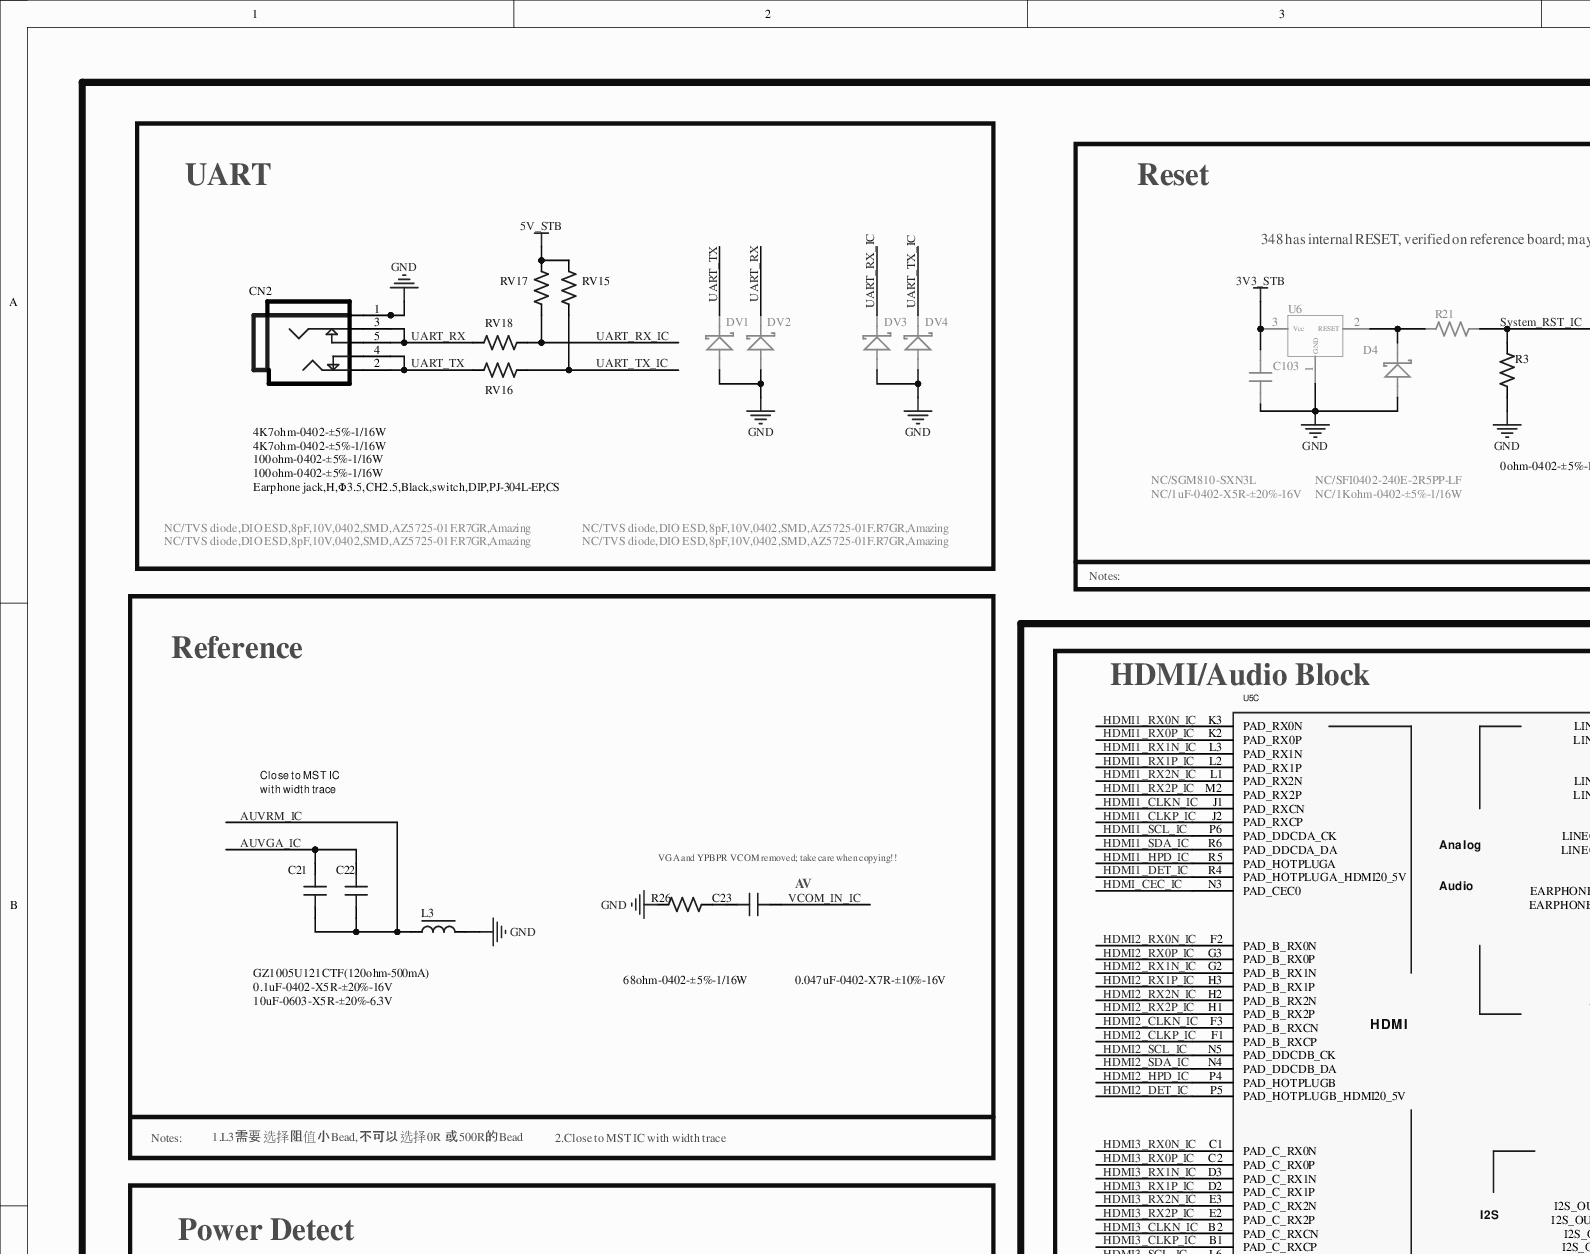
[diagram p0: MISC84395-8.SchDoc, top left]
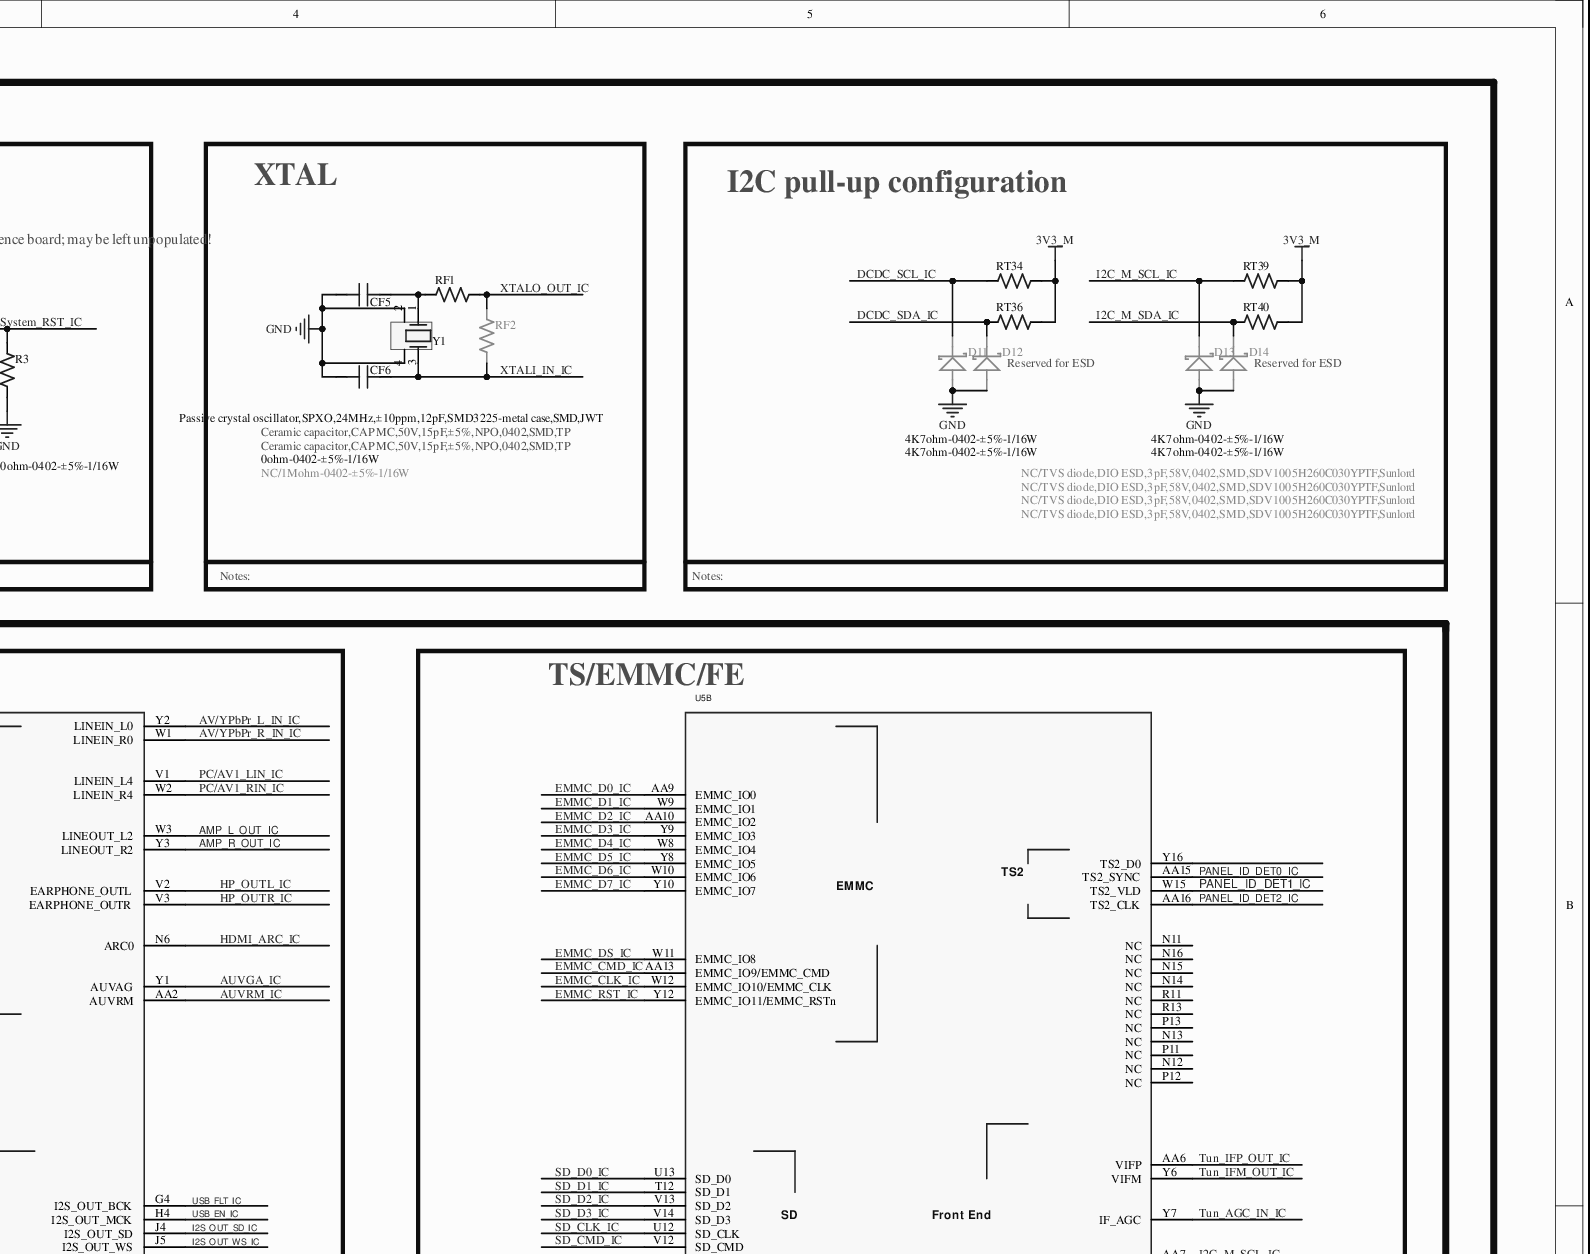
[diagram p1: MISC84395-8.SchDoc, top right]
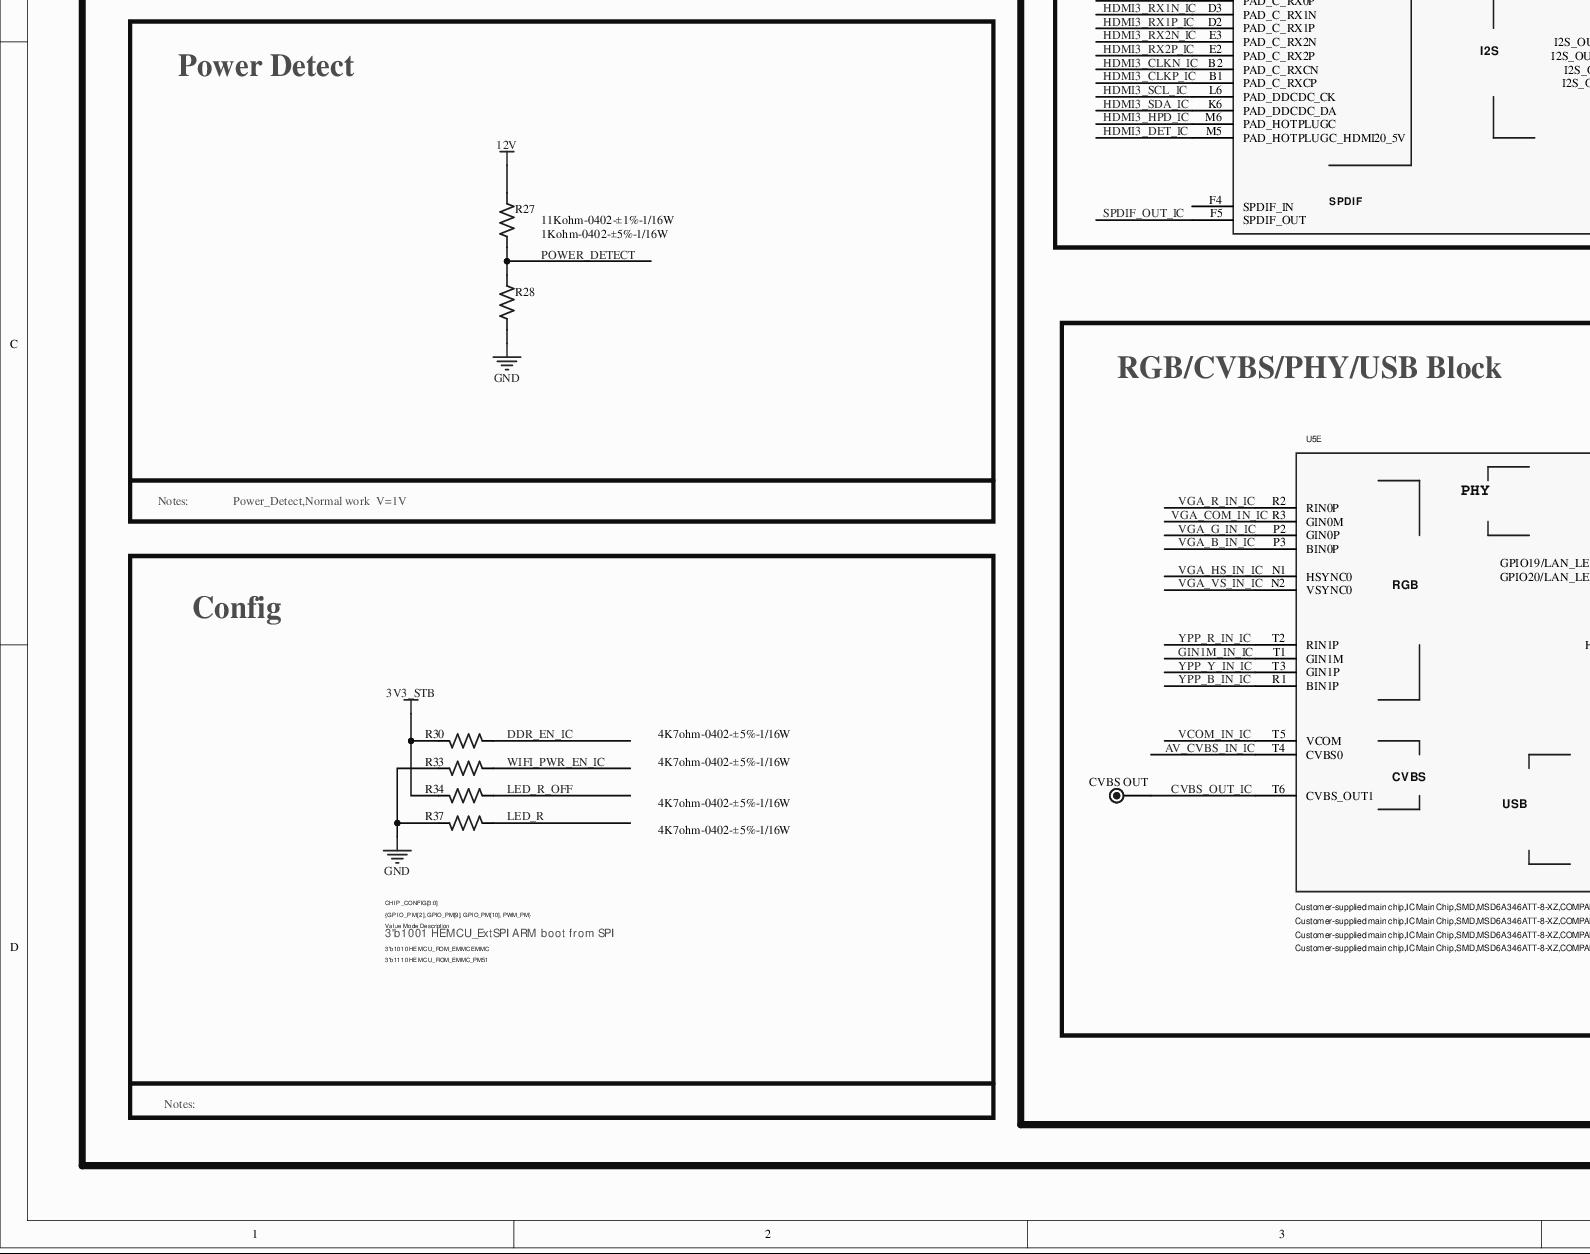
[diagram p2: MISC84395-8.SchDoc, bottom left]
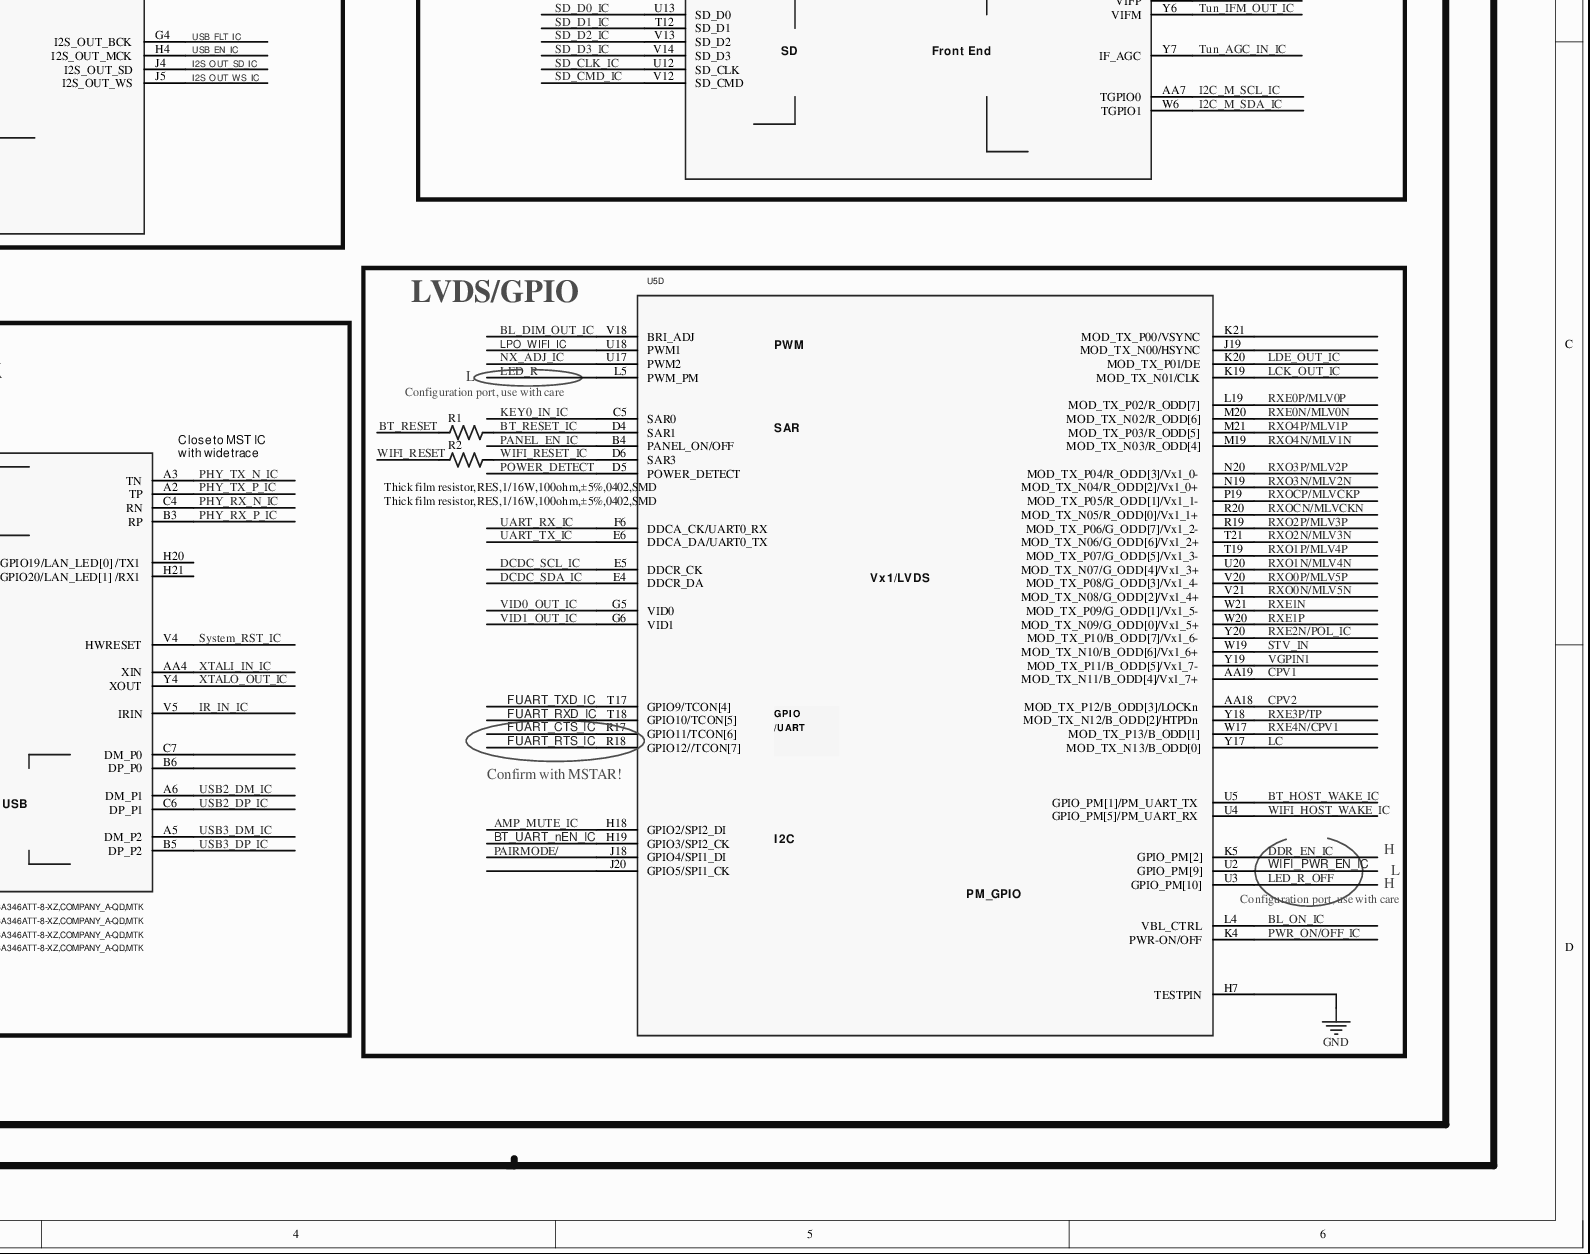
[diagram p3: MISC84395-8.SchDoc, bottom right]
# Altium project MISC84395-37.PrjPCB (part 5 of 13)

## Sheet MISC84395-8.SchDoc
size 571 x 447 mm

### Parts
C21  10uF-0603-X5R-±20%-6.3V  [C0603]
C22  0.1uF-0402-X5R-±20%-16V  [C0402]
C23  0.047uF-0402-X7R-±10%-16V  [C0402]
C103  NC/1uF-0402-X5R-±20%-16V  [C0402]
CF5  Ceramic capacitor,CAP MC,50V,15pF,±5%,NPO,0402,SMD,TP  [C0402]
CF6  Ceramic capacitor,CAP MC,50V,15pF,±5%,NPO,0402,SMD,TP  [C0402]
CN2  Earphone jack,H,Φ3.5,CH2.5,Black,switch,DIP,PJ-304L-EP,CS  [PHONE-HD-54]
CVBS_OUT  TEST  [TP]  (value not drawn)
D4  NC/SFI0402-240E-2R5PP-LF  [DIODE-S0402]
D11  NC/TVS diode,DIO ESD,3pF,58V,0402,SMD,SDV1005H260C030YPTF,Sunlord  [DIODE-S0402]
D12  NC/TVS diode,DIO ESD,3pF,58V,0402,SMD,SDV1005H260C030YPTF,Sunlord  [DIODE-S0402]
D13  NC/TVS diode,DIO ESD,3pF,58V,0402,SMD,SDV1005H260C030YPTF,Sunlord  [DIODE-S0402]
D14  NC/TVS diode,DIO ESD,3pF,58V,0402,SMD,SDV1005H260C030YPTF,Sunlord  [DIODE-S0402]
DV1  NC/TVS diode,DIO ESD,8pF,10V,0402,SMD,AZ5725-01F.R7GR,Amazing  [DIODE-S0402]
DV2  NC/TVS diode,DIO ESD,8pF,10V,0402,SMD,AZ5725-01F.R7GR,Amazing  [DIODE-S0402]
DV3  NC/TVS diode,DIO ESD,8pF,10V,0402,SMD,AZ5725-01F.R7GR,Amazing  [DIODE-S0402]
DV4  NC/TVS diode,DIO ESD,8pF,10V,0402,SMD,AZ5725-01F.R7GR,Amazing  [DIODE-S0402]
L3  GZ1005U121CTF(120ohm-500mA)  [L0402]
R1  Thick film resistor,RES,1/16W,100ohm,±5%,0402,SMD  [R0402]
R2  Thick film resistor,RES,1/16W,100ohm,±5%,0402,SMD  [R0402]
R3  0ohm-0402-±5%-1/16W  [R0402]
R21  NC/1Kohm-0402-±5%-1/16W  [R0402]
R26  68ohm-0402-±5%-1/16W  [R0402]
R27  11Kohm-0402-±1%-1/16W  [R0402]
R28  1Kohm-0402-±5%-1/16W  [R0402]
R30  4K7ohm-0402-±5%-1/16W  [R0402]
R33  4K7ohm-0402-±5%-1/16W  [R0402]
R34  4K7ohm-0402-±5%-1/16W  [R0402]
R37  4K7ohm-0402-±5%-1/16W  [R0402]
RF1  0ohm-0402-±5%-1/16W  [R0402]
RF2  NC/1Mohm-0402-±5%-1/16W  [R0402]
RT34  4K7ohm-0402-±5%-1/16W  [R0402]
RT36  4K7ohm-0402-±5%-1/16W  [R0402]
RT39  4K7ohm-0402-±5%-1/16W  [R0402]
RT40  4K7ohm-0402-±5%-1/16W  [R0402]
RV15  4K7ohm-0402-±5%-1/16W  [R0402]
RV16  100ohm-0402-±5%-1/16W  [R0402]
RV17  4K7ohm-0402-±5%-1/16W  [R0402]
RV18  100ohm-0402-±5%-1/16W  [R0402]
U5  Customer-supplied main chip,IC Main Chip,SMD,MSD6A346ATT-8-XZ,COMPANY_A-QD,MTK  [BGA406/0.8]  (parts B,C,D,E of 7)
U6  NC/SGM810-SXN3L  [SO-23-1]
Y1  Passive crystal oscillator,SPXO,24MHz,±10ppm,12pF,SMD3225-metal case,SMD,JWT  [XTAL-S-3]

### Blocks framed on the sheet
UART: CN2 DV1-DV4 RV15-RV18
Reset: C103 D4 R3 R21 U6
XTAL: CF5 CF6 RF1 RF2 Y1
I2C pull-up configuration: D11-D14 RT34 RT36 RT39 RT40
Reference: C21-C23 L3 R26
HDMI/Audio Block: U5
TS/EMMC/FE: U5
Power Detect: R27 R28
LVDS/GPIO: R1 R2 U5
RGB/CVBS/PHY/USB Block: CVBS_OUT U5
Config: R30 R33 R34 R37

### Nets
3V3_M: RT34.2 RT36.2 RT39.2 RT40.2
3V3_STB: C103.2 R30.1 R34.1 U6.3(Vcc)
5V_STB: RV15.2 RV17.2
12V: R27.2
GND: C103.1 CF5.2 CF6.2 CN2.1 D4.A D11.A D12.A D13.A D14.A DV1.A DV2.A DV3.A DV4.A L3.2 R3.1 R26.1 R28.1 R33.1 R37.1 U5.H7(TESTPIN) U6.1(GND) Y1.2(G) Y1.4
AMP_L_OUT_IC: U5.W3(LINEOUT_L2)
AMP_MUTE_IC: U5.H18(GPIO2/SPI2_DI)
AMP_R_OUT_IC: U5.Y3(LINEOUT_R2)
AUVGA_IC: C21.2 C22.2 U5.Y1(AUVAG)
AUVRM_IC: C21.1 C22.1 L3.1 U5.AA2(AUVRM)
AV/YPbPr_L_IN_IC: U5.Y2(LINEIN_L0)
AV/YPbPr_R_IN_IC: U5.W1(LINEIN_R0)
AV_CVBS_IN_IC: U5.T4(CVBS0)
BL_DIM_OUT_IC: U5.V18(BRI_ADJ)
BL_ON_IC: U5.L4(VBL_CTRL)
BT_HOST_WAKE_IC: U5.U5(GPIO_PM[1]/PM_UART_TX)
BT_RESET: R1.1
BT_RESET_IC: R1.2 U5.D4(SAR1)
BT_UART_nEN_IC: U5.H19(GPIO3/SPI2_CK)
CPV1: U5.AA19(MOD_TX_N11/B_ODD[4]/Vx1_7+)
CPV2: U5.AA18(MOD_TX_P12/B_ODD[3]/LOCKn)
CVBS_OUT_IC: CVBS_OUT.1 U5.T6(CVBS_OUT1)
DCDC_SCL_IC: D11.K RT34.1 U5.E5(DDCR_CK)
DCDC_SDA_IC: D12.K RT36.1 U5.E4(DDCR_DA)
DDR_EN_IC: R30.2 U5.K5(GPIO_PM[2])
EMMC_CLK_IC: U5.W12(EMMC_IO10/EMMC_CLK)
EMMC_CMD_IC: U5.AA13(EMMC_IO9/EMMC_CMD)
EMMC_D0_IC: U5.AA9(EMMC_IO0)
EMMC_D1_IC: U5.W9(EMMC_IO1)
EMMC_D2_IC: U5.AA10(EMMC_IO2)
EMMC_D3_IC: U5.Y9(EMMC_IO3)
EMMC_D4_IC: U5.W8(EMMC_IO4)
EMMC_D5_IC: U5.Y8(EMMC_IO5)
EMMC_D6_IC: U5.W10(EMMC_IO6)
EMMC_D7_IC: U5.Y10(EMMC_IO7)
EMMC_DS_IC: U5.W11(EMMC_IO8)
EMMC_RST_IC: U5.Y12(EMMC_IO11/EMMC_RSTn)
FUART_CTS_IC: U5.R17(GPIO11/TCON[6])
FUART_RTS_IC: U5.R18(GPIO12//TCON[7])
FUART_RXD_IC: U5.T18(GPIO10/TCON[5])
FUART_TXD_IC: U5.T17(GPIO9/TCON[4])
GIN1M_IN_IC: U5.T1(GIN1M)
HDMI1_CLKN_IC: U5.J1(PAD_RXCN)
HDMI1_CLKP_IC: U5.J2(PAD_RXCP)
HDMI1_DET_IC: U5.R4(PAD_HOTPLUGA_HDMI20_5V)
HDMI1_HPD_IC: U5.R5(PAD_HOTPLUGA)
HDMI1_RX0N_IC: U5.K3(PAD_RX0N)
HDMI1_RX0P_IC: U5.K2(PAD_RX0P)
HDMI1_RX1N_IC: U5.L3(PAD_RX1N)
HDMI1_RX1P_IC: U5.L2(PAD_RX1P)
HDMI1_RX2N_IC: U5.L1(PAD_RX2N)
HDMI1_RX2P_IC: U5.M2(PAD_RX2P)
HDMI1_SCL_IC: U5.P6(PAD_DDCDA_CK)
HDMI1_SDA_IC: U5.R6(PAD_DDCDA_DA)
HDMI2_CLKN_IC: U5.F3(PAD_B_RXCN)
HDMI2_CLKP_IC: U5.F1(PAD_B_RXCP)
HDMI2_DET_IC: U5.P5(PAD_HOTPLUGB_HDMI20_5V)
HDMI2_HPD_IC: U5.P4(PAD_HOTPLUGB)
HDMI2_RX0N_IC: U5.F2(PAD_B_RX0N)
HDMI2_RX0P_IC: U5.G3(PAD_B_RX0P)
HDMI2_RX1N_IC: U5.G2(PAD_B_RX1N)
HDMI2_RX1P_IC: U5.H3(PAD_B_RX1P)
HDMI2_RX2N_IC: U5.H2(PAD_B_RX2N)
HDMI2_RX2P_IC: U5.H1(PAD_B_RX2P)
HDMI2_SCL_IC: U5.N5(PAD_DDCDB_CK)
HDMI2_SDA_IC: U5.N4(PAD_DDCDB_DA)
HDMI3_CLKN_IC: U5.B2(PAD_C_RXCN)
HDMI3_CLKP_IC: U5.B1(PAD_C_RXCP)
HDMI3_DET_IC: U5.M5(PAD_HOTPLUGC_HDMI20_5V)
HDMI3_HPD_IC: U5.M6(PAD_HOTPLUGC)
HDMI3_RX0N_IC: U5.C1(PAD_C_RX0N)
HDMI3_RX0P_IC: U5.C2(PAD_C_RX0P)
HDMI3_RX1N_IC: U5.D3(PAD_C_RX1N)
HDMI3_RX1P_IC: U5.D2(PAD_C_RX1P)
HDMI3_RX2N_IC: U5.E3(PAD_C_RX2N)
HDMI3_RX2P_IC: U5.E2(PAD_C_RX2P)
HDMI3_SCL_IC: U5.L6(PAD_DDCDC_CK)
HDMI3_SDA_IC: U5.K6(PAD_DDCDC_DA)
HDMI_ARC_IC: U5.N6(ARC0)
HDMI_CEC_IC: U5.N3(PAD_CEC0)
HP_OUTL_IC: U5.V2(EARPHONE_OUTL)
HP_OUTR_IC: U5.V3(EARPHONE_OUTR)
I2C_M_SCL_IC: D13.K RT39.1 U5.AA7(TGPIO0)
I2C_M_SDA_IC: D14.K RT40.1 U5.W6(TGPIO1)
I2S_OUT_SD_IC: U5.J4(I2S_OUT_SD)
I2S_OUT_WS_IC: U5.J5(I2S_OUT_WS)
IR_IN_IC: U5.V5(IRIN)
KEY0_IN_IC: U5.C5(SAR0)
LC: U5.Y17(MOD_TX_N13/B_ODD[0])
LCK_OUT_IC: U5.K19(MOD_TX_N01/CLK)
LDE_OUT_IC: U5.K20(MOD_TX_P01/DE)
LED_R: R37.2 U5.L5(PWM_PM)
LED_R_OFF: R34.2 U5.U3(GPIO_PM[10])
LPO_WIFI_IC: U5.U18(PWM1)
NX_ADJ_IC: U5.U17(PWM2)
PAIRMODE/: U5.J18(GPIO4/SPI1_DI)
PANEL_EN_IC: U5.B4(PANEL_ON/OFF)
PANEL_ID_DET0_IC: U5.AA15(TS2_SYNC)
PANEL_ID_DET1_IC: U5.W15(TS2_VLD)
PANEL_ID_DET2_IC: U5.AA16(TS2_CLK)
PC/AV1_LIN_IC: U5.V1(LINEIN_L4)
PC/AV1_RIN_IC: U5.W2(LINEIN_R4)
PHY_RX_N_IC: U5.C4(RN)
PHY_RX_P_IC: U5.B3(RP)
PHY_TX_N_IC: U5.A3(TN)
PHY_TX_P_IC: U5.A2(TP)
POWER_DETECT: R27.1 R28.2 U5.D5(POWER_DETECT)
PWR_ON/OFF_IC: U5.K4(PWR-ON/OFF)
RXE0N/MLV0N: U5.M20(MOD_TX_N02/R_ODD[6])
RXE0P/MLV0P: U5.L19(MOD_TX_P02/R_ODD[7])
RXE1N: U5.W21(MOD_TX_P09/G_ODD[1]/Vx1_5-)
RXE1P: U5.W20(MOD_TX_N09/G_ODD[0]/Vx1_5+)
RXE2N/POL_IC: U5.Y20(MOD_TX_P10/B_ODD[7]/Vx1_6-)
RXE3P/TP: U5.Y18(MOD_TX_N12/B_ODD[2]/HTPDn)
RXE4N/CPV1: U5.W17(MOD_TX_P13/B_ODD[1])
RXO0N/MLV5N: U5.V21(MOD_TX_N08/G_ODD[2]/Vx1_4+)
RXO0P/MLV5P: U5.V20(MOD_TX_P08/G_ODD[3]/Vx1_4-)
RXO1N/MLV4N: U5.U20(MOD_TX_N07/G_ODD[4]/Vx1_3+)
RXO1P/MLV4P: U5.T19(MOD_TX_P07/G_ODD[5]/Vx1_3-)
RXO2N/MLV3N: U5.T21(MOD_TX_N06/G_ODD[6]/Vx1_2+)
RXO2P/MLV3P: U5.R19(MOD_TX_P06/G_ODD[7]/Vx1_2-)
RXO3N/MLV2N: U5.N19(MOD_TX_N04/R_ODD[2]/Vx1_0+)
RXO3P/MLV2P: U5.N20(MOD_TX_P04/R_ODD[3]/Vx1_0-)
RXO4N/MLV1N: U5.M19(MOD_TX_N03/R_ODD[4])
RXO4P/MLV1P: U5.M21(MOD_TX_P03/R_ODD[5])
RXOCN/MLVCKN: U5.R20(MOD_TX_N05/R_ODD[0]/Vx1_1+)
RXOCP/MLVCKP: U5.P19(MOD_TX_P05/R_ODD[1]/Vx1_1-)
SD_CLK_IC: U5.U12(SD_CLK)
SD_CMD_IC: U5.V12(SD_CMD)
SD_D0_IC: U5.U13(SD_D0)
SD_D1_IC: U5.T12(SD_D1)
SD_D2_IC: U5.V13(SD_D2)
SD_D3_IC: U5.V14(SD_D3)
SPDIF_OUT_IC: U5.F5(SPDIF_OUT)
STV_IN: U5.W19(MOD_TX_N10/B_ODD[6]/Vx1_6+)
System_RST_IC: R3.2 R21.1 U5.V4(HWRESET)
Tun_AGC_IN_IC: U5.Y7(IF_AGC)
Tun_IFM_OUT_IC: U5.Y6(VIFM)
Tun_IFP_OUT_IC: U5.AA6(VIFP)
UART_RX: CN2.3 CN2.5 DV2.K RV18.1
UART_RX_IC: DV3.K RV17.1 RV18.2 U5.F6(DDCA_CK/UART0_RX)
UART_TX: CN2.2 CN2.4 DV1.K RV16.2
UART_TX_IC: DV4.K RV15.1 RV16.1 U5.E6(DDCA_DA/UART0_TX)
USB2_DM_IC: U5.A6(DM_P1)
USB2_DP_IC: U5.C6(DP_P1)
USB3_DM_IC: U5.A5(DM_P2)
USB3_DP_IC: U5.B5(DP_P2)
USB_EN_IC: U5.H4(I2S_OUT_MCK)
USB_FLT_IC: U5.G4(I2S_OUT_BCK)
VCOM_IN_IC: C23.1 U5.T5(VCOM)
VGA_B_IN_IC: U5.P3(BIN0P)
VGA_COM_IN_IC: U5.R3(GIN0M)
VGA_G_IN_IC: U5.P2(GIN0P)
VGA_HS_IN_IC: U5.N1(HSYNC0)
VGA_R_IN_IC: U5.R2(RIN0P)
VGA_VS_IN_IC: U5.N2(VSYNC0)
VGPIN1: U5.Y19(MOD_TX_P11/B_ODD[5]/Vx1_7-)
VID0_OUT_IC: U5.G5(VID0)
VID1_OUT_IC: U5.G6(VID1)
WIFI_HOST_WAKE_IC: U5.U4(GPIO_PM[5]/PM_UART_RX)
WIFI_PWR_EN_IC: R33.2 U5.U2(GPIO_PM[9])
WIFI_RESET: R2.1
WIFI_RESET_IC: R2.2 U5.D6(SAR3)
XTALI_IN_IC: CF6.1 RF2.1 U5.AA4(XIN) Y1.3
XTALO_OUT_IC: RF1.2 RF2.2 U5.Y4(XOUT)
YPP_B_IN_IC: U5.R1(BIN1P)
YPP_R_IN_IC: U5.T2(RIN1P)
YPP_Y_IN_IC: U5.T3(GIN1P)
NetC23_2: C23.2 R26.2
NetCF5_1: CF5.1 RF1.1 Y1.1
NetD4_K: D4.K R21.2 U6.2(RESET)

Not connected (* = marked no-connect by the designer): U5 B6(DP_P0)* C7(DM_P0)* F4(SPDIF_IN)* H20(GPIO19/LAN_LED[0]_/TX1)* H21(GPIO20/LAN_LED[1]_/RX1)* J19(MOD_TX_N00/HSYNC)* J20(GPIO5/SPI1_CK)* K21(MOD_TX_P00/VSYNC)* N11(NC)* N12(NC)* N13(NC)* N14(NC)* N15(NC)* N16(NC)* P11(NC)* P12(NC)* P13(NC)* R11(NC)* R13(NC)* Y16(TS2_D0)*

### Notes on the sheet
- (near CF5) 348 has internal RESET, verified on reference board; may be left unpopulated!
- Reserved for ESD
- Notes:
- Close to MST IC
- with width trace
- VGA and YPBPR VCOM removed; take care when copying!!
- (near C23) AV
- 1.L3需要选择阻值小Bead,不可以选择0R 或500R的Bead
- 2.Close to MST IC with width trace
- L
- (near U5) Close to MST IC
- (near U5) with wide trace
- Configuration port, use with care
- Power_Detect,Normal work   V=1V
- (near U5) Confirm with MSTAR!
- H
- CHIP_CONFIG[3:0]
- {GPIO_PM[2],GPIO_PM[9], GPIO_PM[10], PWM_PM}
- Value Mode Description
- (near U5) Configuration port, use with care
- 3'b1001 HEMCU_ExtSPI ARM boot from SPI
- 3'b1010 HEMCU_ROM_EMMC EMMC
- 3'b1110 HEMCU_ROM_EMMC_PM51

### Library data of the parts
C21 = 10uF-0603-X5R-±20%-6.3V-D
C22 C103 = 0.1uF-0402-X5R-±20%-16V-D
C23 = 0.047uF-0402-X7R-±10%-16V-D
CF5 CF6 = 33pF-0402-NPO-±5%-50V-D
CN2 = XXX.XXX.0004738-DLMI: Earphone jack,H,Φ3.5,CH2.5,Black,switch,DIP,PJ-304L-EP,CS-DLMI
D4 = SFI0402-240E-2R5PP-LF-D
D11-D14 DV1-DV4 = AVLC18S02003-D
L3 = GZ1005U121CTF(120ohm-500mA)-D
R1 R2 = 004.002.0000568-D: Thick film resistor,RES,1/16W,100ohm,±5%,0402,SMD-D
R3 RF1 = 0ohm-0402-±5%-1/16W-D
R21 R28 = 1Kohm-0402-±5%-1/16W-D
R26 = 180ohm-0402-±5%-1/16W-D
R27 = 11Kohm-0402-±1%-1/16W-D
R30 R33 R34 R37 RT34 RT36 RT39 RT40 RV15 RV17 = 4K7ohm-0402-±5%-1/16W-D
RF2 = 1Mohm-0402-±5%-1/16W-D
RV16 RV18 = 100ohm-0402-±5%-1/16W-D
U5 = 004.016.0000830: TV main chip,IC Main Chip,MSD6A348AT-X1,CAN TV,32bit,Multi-Core,BGA406,SMD,Mstar-D
U6 = SGM810-SXN3L-D
Y1 = 32MHz-±10PPM-12PF-SMD3225-JWT-D